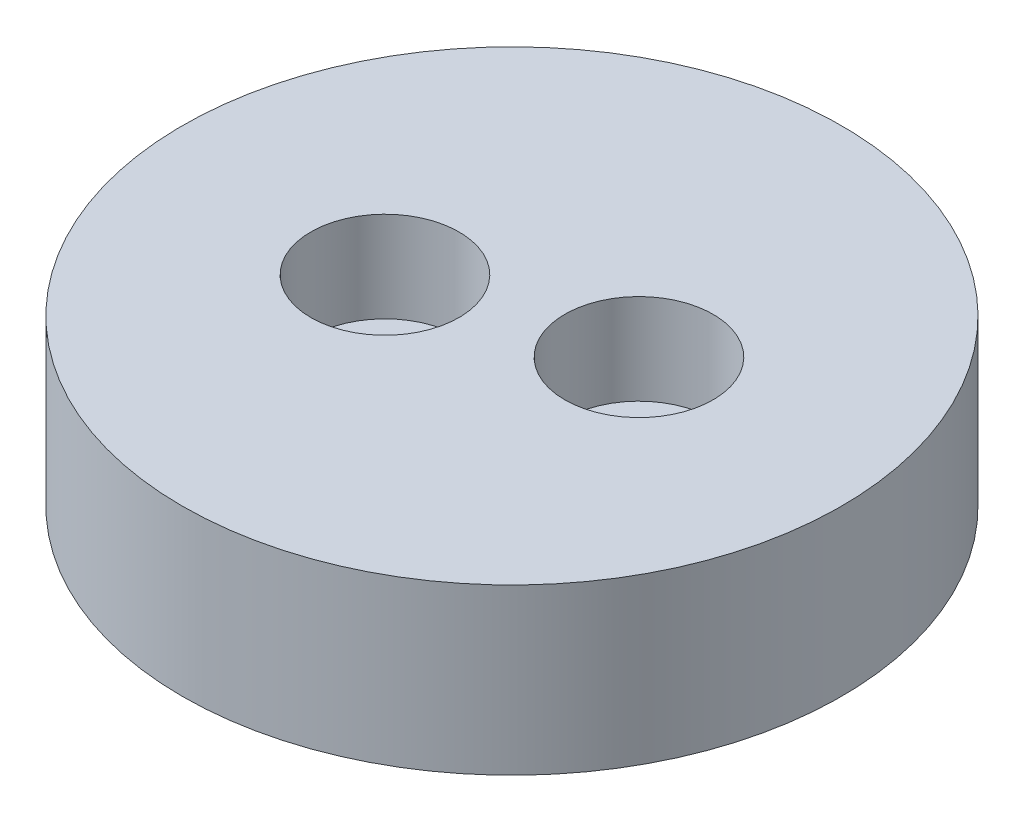
from build123d import *

# Parameters (mm, degrees)
SKETCH1_R                                           = 40
BOSS_EXTRUDE1_DEPTH                                 = 20
HOLE_SIZE_PER_SOCKET_HEAD_CAP_SCREW_TYP_D           = 11
HOLE_SIZE_PER_SOCKET_HEAD_CAP_SCREW_TYP_CBORE_D     = 18
HOLE_SIZE_PER_SOCKET_HEAD_CAP_SCREW_TYP_CBORE_DEPTH = 11


with BuildPart() as part:
    # Sketch1 → Boss-Extrude1 (new body)
    with BuildSketch(Plane(origin=(0, 0, 0), x_dir=(1, 0, 0), z_dir=(0, 1, 0))):
        with Locations(Location((0, 0, 0), (0, 0, 270))):
            Circle(SKETCH1_R)
    extrude(amount=BOSS_EXTRUDE1_DEPTH)

    # Hole size (per socket head cap screw type) 1 (through all)
    with Locations(Plane(origin=(-12.034248035, 20, 3.380365992), x_dir=(0, 0, 1), z_dir=(0, 1, 0))):
        with Locations((0, 0), (-6.760731984, 24.06849607)):
            CounterBoreHole(HOLE_SIZE_PER_SOCKET_HEAD_CAP_SCREW_TYP_D / 2, HOLE_SIZE_PER_SOCKET_HEAD_CAP_SCREW_TYP_CBORE_D / 2, HOLE_SIZE_PER_SOCKET_HEAD_CAP_SCREW_TYP_CBORE_DEPTH)


solid = part.part
